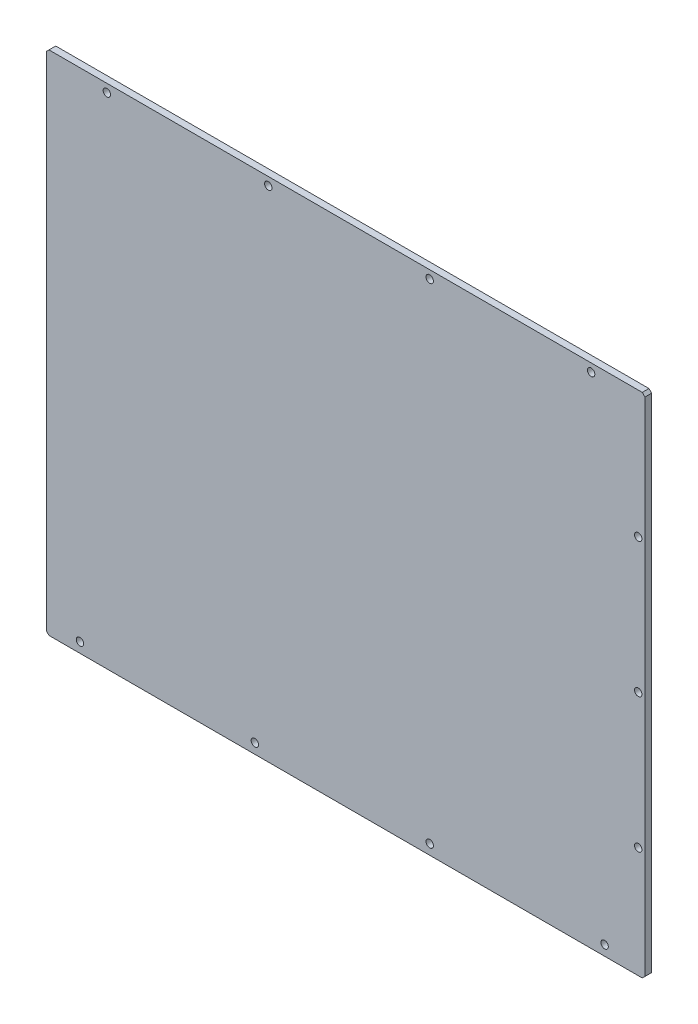
SolidWorks part; units mm, degrees
material "PC "
ref_plane "Front Plane" through (0, 0, 0) normal (0, 0, 1) x (1, 0, 0)
ref_plane "Top Plane" through (0, 0, 0) normal (0, 1, 0) x (1, 0, 0)
ref_plane "Right Plane" through (0, 0, 0) normal (1, 0, 0) x (0, 0, -1)
sketch "Sketch1" plane through (0, 0, 0) normal (0, 0, 1) x (1, 0, 0)
  line L1 (-222.5, 188.5) -> (222.5, 188.5)
  line L2 (-222.5, 188.5) -> (-222.5, -188.5)
  line L3 (-222.5, -188.5) -> (222.5, -188.5)
  line L4 (222.5, 188.5) -> (222.5, -188.5)
  line L5 (-222.5, 188.5) -> (222.5, -188.5) construction
  line L6 (-222.5, -188.5) -> (222.5, 188.5) construction
  point P0 (0, 0)
  dimension "D1" = 377
  dimension "D2" = 445
extrude "Boss-Extrude1" add sketch "Sketch1" along normal blind 5
hole_wizard "M5 Clearance Hole1" positions "Sketch2" profile "Sketch3" hole size "M5" standard "GB" end condition through all
sketch "Sketch2" plane through (0, 0, 5) normal (0, 0, 1) x (1, 0, 0)
  point P107 (-177.5, 182.5)
  point P110 (-57.5, 182.5)
  point P113 (62.5, 182.5)
  point P116 (182.5, 182.5)
  point P119 (-197.5, -181)
  point P122 (-67.5, -181)
  point P125 (62.5, -181)
  point P128 (192.5, -181)
  point P131 (217.5, -106)
  point P134 (217.5, -6)
  point P137 (217.5, 94)
sketch "Sketch3" plane through (-177.5, 182.5, 5) normal (1, 0, 0) x (0, -1, 0)
  line L0 (0, 0) -> (0, 5)
  line L1 (0, 5) -> (2.75, 5)
  line L2 (2.75, 5) -> (2.75, 0)
  line L5 (2.75, 0) -> (0, 0)
  line L11 (0, -6.35) -> (0, 107.95) construction
  dimension "通孔孔直径" = 5.5
  dimension "通孔孔深度" = 5
fillet "Fillet1" radius 2 4 edges at (222.5, -188.5, 2.5) (-222.5, -188.5, 2.5) (-222.5, 188.5, 2.5) (222.5, 188.5, 2.5) profile chamfer
